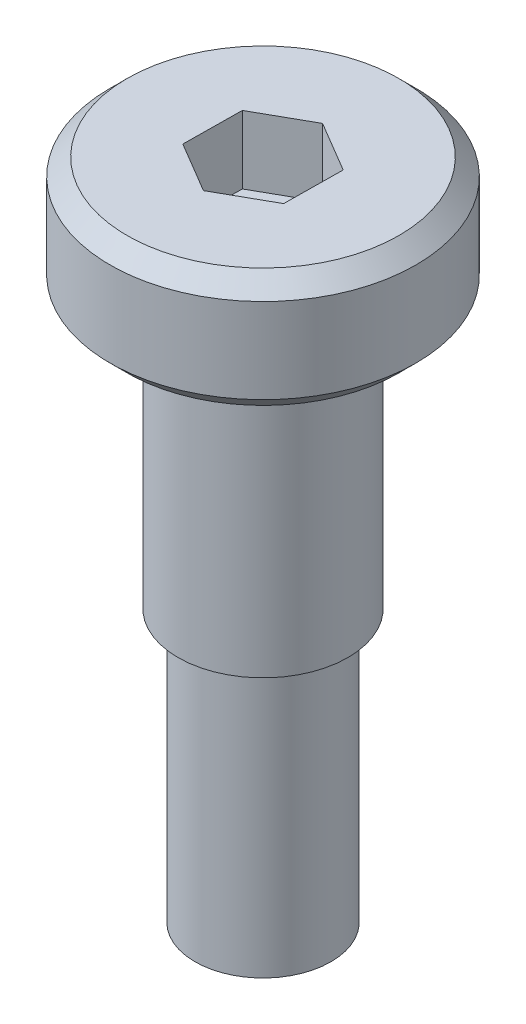
SolidWorks part; units mm, degrees
ref_plane "Front Plane" through (0, 0, 0) normal (0, 0, 1) x (1, 0, 0)
ref_plane "Top Plane" through (0, 0, 0) normal (0, 1, 0) x (1, 0, 0)
ref_plane "Right Plane" through (0, 0, 0) normal (1, 0, 0) x (0, 0, -1)
sketch "Sketch1" plane through (0, 0, 0) normal (0, 0, 1) x (1, 0, 0)
  line L0 (0, 0) -> (0, 19.5)
  line L1 (0, 19.5) -> (-4.5, 19.5)
  line L2 (-4.5, 19.5) -> (-4.5, 16)
  line L3 (-4.5, 16) -> (-2.5, 16)
  line L4 (-2.5, 16) -> (-2.5, 8)
  line L5 (-2.5, 8) -> (-2, 8)
  line L6 (-2, 8) -> (-2, 0)
  line L7 (-2, 0) -> (0, 0)
  dimension "D1" = 2
  dimension "D2" = 8
  dimension "D3" = 2.5
  dimension "D4" = 8
  dimension "D5" = 4.5
  dimension "D6" = 3.5
revolve "Revolve1" add sketch "Sketch1" angle 360 about L0
sketch "Sketch2" plane through (0, 19.5, 0) normal (0, 1, 0) x (1, 0, 0)
  line L1 (1.5096, 0.8492) -> (0.0193, 1.7319)
  line L2 (0.0193, 1.7319) -> (-1.4902, 0.8827)
  line L3 (-1.4902, 0.8827) -> (-1.5096, -0.8492)
  line L4 (-1.5096, -0.8492) -> (-0.0193, -1.7319)
  line L5 (-0.0193, -1.7319) -> (1.4902, -0.8827)
  line L6 (1.4902, -0.8827) -> (1.5096, 0.8492)
  circle A0 centre (0, 0) radius 1.5 construction
  dimension "D1" = 3
extrude "Cut-Extrude1" cut sketch "Sketch2" against normal blind 2
chamfer "Chamfer1" distance 0.5 angle 45 2 edges at (4.5, 16, 0) (4.5, 19.5, 0)
